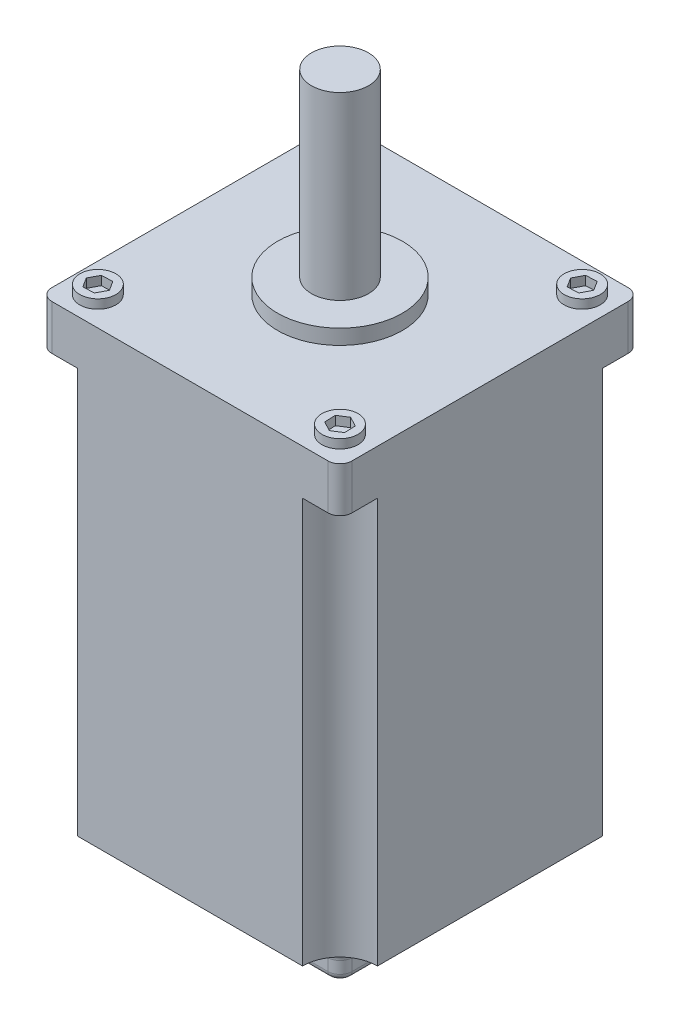
SolidWorks part; units mm, degrees
ref_plane "Front Plane" through (0, 0, 0) normal (0, 0, 1) x (1, 0, 0)
ref_plane "Top Plane" through (0, 0, 0) normal (0, 1, 0) x (1, 0, 0)
ref_plane "Right Plane" through (0, 0, 0) normal (1, 0, 0) x (0, 0, -1)
other "Configuration Table"
sketch "Sketch1" plane through (0, 0, 0) normal (0, 1, 0) x (1, 0, 0)
  circle A0 centre (0, 0) radius 9.5
  dimension "D1" = 19
extrude "Boss-Extrude1" add sketch "Sketch1" along normal blind 60
sketch "Sketch2" plane through (0, 0, 0) normal (0, -1, 0) x (1, 0, 0)
  circle A0 centre (0, 0) radius 20.7926
extrude "Boss-Extrude2" add sketch "Sketch2" along normal blind 5
sketch "Sketch3" plane through (0, -5, 0) normal (0, -1, 0) x (1, 0, 0)
  line L1 (-50, 50) -> (50, 50)
  line L2 (-50, 50) -> (-50, -50)
  line L3 (-50, -50) -> (50, -50)
  line L4 (50, 50) -> (50, -50)
  line L5 (-50, 50) -> (50, -50) construction
  line L6 (-50, -50) -> (50, 50) construction
  point P0 (0, 0)
  dimension "D1" = 100
extrude "Boss-Extrude3" add sketch "Sketch3" along normal blind 150
sketch "Sketch4" plane through (0, -155, 0) normal (0, -1, 0) x (1, 0, 0)
  circle A0 centre (-50, 50) radius 12.5
  circle A1 centre (50, 50) radius 12.5
  circle A2 centre (-50, -50) radius 12.5
  circle A3 centre (50, -50) radius 12.5
  dimension "D1" = 25
extrude "Cut-Extrude1" cut sketch "Sketch4" against normal blind 135
fillet "Fillet1" radius 4 4 edges at (50, -12.5, 50) (50, -12.5, -50) (-50, -12.5, -50) (-50, -12.5, 50)
sketch "Sketch5" plane through (0, -155, 0) normal (0, -1, 0) x (1, 0, 0)
  line L5 (-39.3533, 39.3533) -> (39.3533, 39.3533)
  line L6 (-39.3533, 39.3533) -> (-39.3533, -39.3533)
  line L7 (-39.3533, -39.3533) -> (39.3533, -39.3533)
  line L8 (39.3533, 39.3533) -> (39.3533, -39.3533)
  line L9 (-39.3533, 39.3533) -> (39.3533, -39.3533) construction
  line L10 (-39.3533, -39.3533) -> (39.3533, 39.3533) construction
  point P0 (0, 0)
extrude "Boss-Extrude4" add sketch "Sketch5" along normal blind 10
fillet "Fillet2" radius 4 8 edges at (39.3533, -155, 0) (39.3533, -160, 39.3533) (0, -155, 39.3533) (-39.3533, -160, 39.3533) (-39.3533, -155, 0) (-39.3533, -160, -39.3533) (0, -155, -39.3533) (39.3533, -160, -39.3533)
fillet "Fillet3" radius 2 8 edges at (38.1817, -165, -38.1817) (0, -165, -39.3533) (-38.1817, -165, -38.1817) (-39.3533, -165, 0) (-38.1817, -165, 38.1817) (0, -165, 39.3533) (38.1817, -165, 38.1817) (39.3533, -165, 0)
sketch "Sketch6" plane through (0, 0, 0) normal (0, 0, 1) x (1, 0, 0)
  line L0 (35.3533, -165) -> (-35.3533, -165) construction
  line L1 (-33.7334, -169.5966) -> (33.7334, -169.5966)
  line L2 (-33.7334, -169.5966) -> (-33.7334, -160.4034)
  line L3 (-33.7334, -160.4034) -> (33.7334, -160.4034)
  line L4 (33.7334, -169.5966) -> (33.7334, -160.4034)
  line L5 (-33.7334, -169.5966) -> (33.7334, -160.4034) construction
  line L6 (-33.7334, -160.4034) -> (33.7334, -169.5966) construction
  point P0 (0, -165)
extrude "Cut-Extrude2" cut sketch "Sketch6" against normal blind 1.5 and the other way blind 1.5
pattern_linear "LPattern1" count 6 spacing 6.5 along (0, 0, 1) count 6 spacing 6.5 along (0, 0, -1) seed only of "Cut-Extrude2"
sketch "Sketch7" plane through (0, -5, 0) normal (0, 1, 0) x (1, 0, 0)
  line L0 (-48.8284, 48.8284) -> (48.8284, -48.8284) construction
  line L2 (-37.0684, 38.6229) -> (-37.216, 42.3191)
  line L3 (-37.216, 42.3191) -> (-40.4908, 44.0393)
  line L4 (-40.4908, 44.0393) -> (-43.6179, 42.0633)
  line L5 (-43.6179, 42.0633) -> (-43.4703, 38.3672)
  line L6 (-43.4703, 38.3672) -> (-40.1955, 36.647)
  line L7 (-40.1955, 36.647) -> (-37.0684, 38.6229)
  arc A0 (-46, 50) -> (-50, 46) centre (-46, 46) ccw construction
  arc A1 (46, -50) -> (50, -46) centre (46, -46) ccw construction
  circle A2 centre (-40.3431, 40.3431) radius 6
  circle A3 centre (-40.3431, 40.3431) radius 3.2035 construction
  dimension "D2" = 12
  dimension "D1" = 12
extrude "Boss-Extrude5" add sketch "Sketch7" along normal blind 3
pattern_circular "CirPattern1" count 4 over 360 about axis through (0, 0, 0) along (0, 1, 0) of "Boss-Extrude5"
